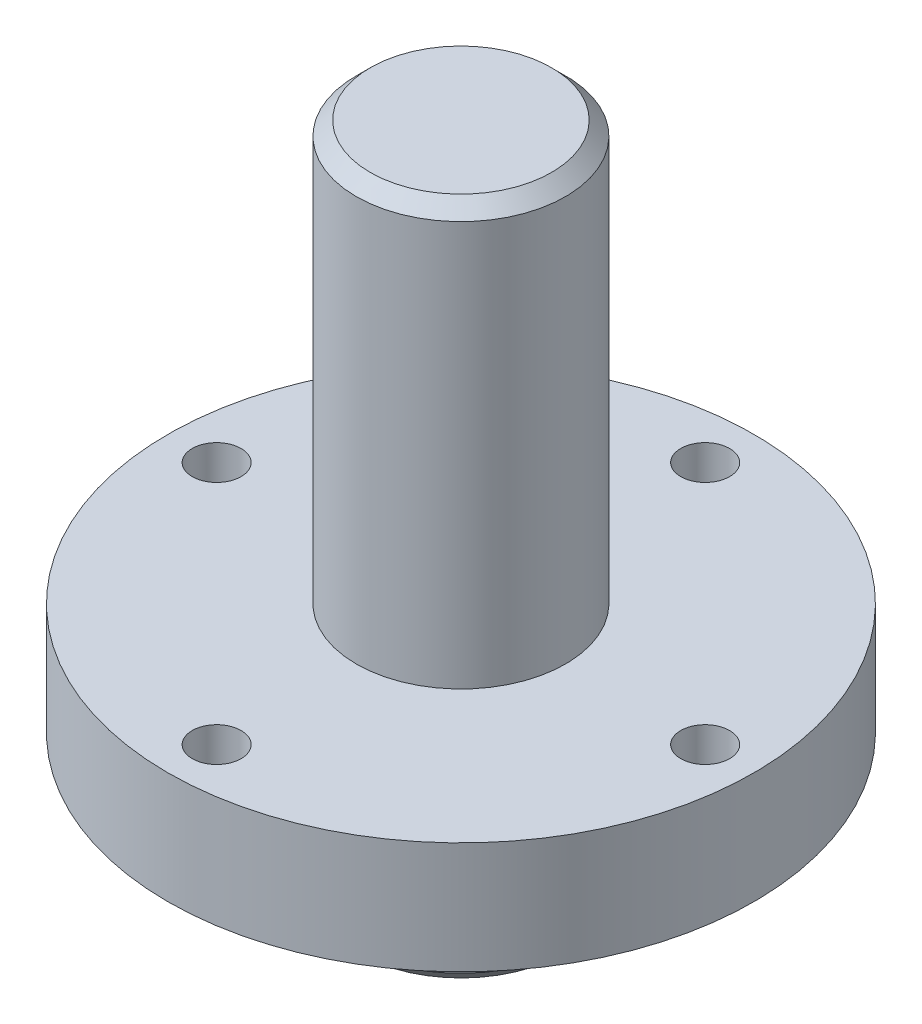
from build123d import *

# Parameters (mm, degrees)
SKETCH1_R           = 15
BOSS_EXTRUDE1_DEPTH = 65
SKETCH2_R           = 14
BOSS_EXTRUDE2_DEPTH = 260
SKETCH3_W           = 22.007775422
SKETCH3_H           = 2
CUT_EXTRUDE1_DEPTH  = 22
CIRPATTERN1_COUNT   = 4
SKETCH4_R           = 10.5
BOSS_EXTRUDE3_DEPTH = 30
SKETCH5_R           = 10.3
BOSS_EXTRUDE4_DEPTH = 10
SKETCH6_R           = 10.5
BOSS_EXTRUDE5_DEPTH = 16
CHAMFER1_SIZE       = 8
CHAMFER1_SIZE2      = 1
SKETCH8_R           = 7.5
BOSS_EXTRUDE6_DEPTH = 30
BOSS_EXTRUDE7_START = -8
SKETCH11_R          = 21
SKETCH11_R_2        = 15
BOSS_EXTRUDE7_DEPTH = 8
SKETCH13_R          = 19
CUT_EXTRUDE4_DEPTH  = 373
SKETCH14_R          = 8.4
BOSS_EXTRUDE8_DEPTH = 10
CHAMFER3_SIZE       = 1
SKETCH16_R          = 1.75
CUT_EXTRUDE5_DEPTH  = 43.213741838
CIRPATTERN3_COUNT   = 4


with BuildPart() as part:
    # Sketch1 → Boss-Extrude1 (new body)
    with BuildSketch(Plane(origin=(0, 0, 0), x_dir=(1, 0, 0), z_dir=(0, 1, 0))):
        with Locations(Location((0, 0, 0), (0, 0, 270))):
            Circle(SKETCH1_R)
    extrude(amount=BOSS_EXTRUDE1_DEPTH)

    # Sketch2 → Boss-Extrude2 (add)
    with BuildSketch(Plane.XZ):
        with Locations(Location((0, 0, 0), (0, 0, 90))):
            Circle(SKETCH2_R)
    extrude(amount=BOSS_EXTRUDE2_DEPTH)

    # Sketch3 → Cut-Extrude1 (cut)
    with BuildSketch(Plane.XZ.offset(260)):
        with Locations((0, -14)):
            Rectangle(SKETCH3_W, SKETCH3_H)
        with Locations((0, 14)):
            Rectangle(SKETCH3_W, SKETCH3_H)
    cut_extrude1 = extrude(amount=-CUT_EXTRUDE1_DEPTH, mode=Mode.SUBTRACT)

    # CirPattern1: Cut-Extrude1 ×4 about axis
    cirpattern1_axis = Axis((0, -260, 0), (0, 1, 0))
    for i in range(1, CIRPATTERN1_COUNT):
        add(cut_extrude1.rotate(cirpattern1_axis, i * 360 / CIRPATTERN1_COUNT), mode=Mode.SUBTRACT)

    # Sketch4 → Boss-Extrude3 (add)
    with BuildSketch(Plane.XZ.offset(260)):
        with Locations(Location((0, 0, 0), (0, 0, 270))):
            Circle(SKETCH4_R)
    extrude(amount=BOSS_EXTRUDE3_DEPTH)

    # Sketch5 → Boss-Extrude4 (add)
    with BuildSketch(Plane.XZ.offset(290)):
        with Locations(Location((0, 0, 0), (0, 0, 270))):
            Circle(SKETCH5_R)
    extrude(amount=BOSS_EXTRUDE4_DEPTH)

    # Sketch6 → Boss-Extrude5 (add)
    with BuildSketch(Plane.XZ.offset(300)):
        with Locations(Location((0, 0, 0), (0, 0, 270))):
            Circle(SKETCH6_R)
    extrude(amount=BOSS_EXTRUDE5_DEPTH)

    # Chamfer1
    chamfer1_edges = [part.edges().sort_by_distance(p)[0] for p in [
        (0, -316, 10.5),
    ]]
    chamfer1_side = [part.faces().sort_by_distance(p)[0] for p in [
        (0, -308, 10.5),
    ]]
    chamfer(chamfer1_edges, length=CHAMFER1_SIZE, length2=CHAMFER1_SIZE2, reference=chamfer1_side[0])

    # Sketch8 → Boss-Extrude6 (add)
    with BuildSketch(Plane(origin=(0, 65, 0), x_dir=(1, 0, 0), z_dir=(0, 1, 0))):
        with Locations(Location((0, 0, 0), (0, 0, 270))):
            Circle(SKETCH8_R)
    extrude(amount=BOSS_EXTRUDE6_DEPTH)

    # Sketch11 → Boss-Extrude7 (add)
    with BuildSketch(Plane(origin=(0, 65, 0), x_dir=(1, 0, 0), z_dir=(0, 1, 0)).offset(BOSS_EXTRUDE7_START)):
        with Locations(Location((0, 0, 0), (0, 0, 270))):
            Circle(SKETCH11_R)
        with Locations(Location((0, 0, 0), (0, 0, 270))):
            Circle(SKETCH11_R_2, mode=Mode.SUBTRACT)
    extrude(amount=BOSS_EXTRUDE7_DEPTH)

    # Sketch13 → Cut-Extrude4 (cut)
    with BuildSketch(Plane.XZ.offset(316)):
        Circle(SKETCH13_R)
    extrude(amount=-CUT_EXTRUDE4_DEPTH, mode=Mode.SUBTRACT)

    # Sketch14 → Boss-Extrude8 (add)
    with BuildSketch(Plane.XZ.offset(-57)):
        with Locations(Location((0, 0, 0), (0, 0, 90))):
            Circle(SKETCH14_R)
    extrude(amount=BOSS_EXTRUDE8_DEPTH)

    # Chamfer3
    chamfer3_edges = [part.edges().sort_by_distance(p)[0] for p in [
        (0, 95, -7.5),
        (0, 47, -8.4),
    ]]
    chamfer(chamfer3_edges, length=CHAMFER3_SIZE)

    # Sketch16 → Cut-Extrude5 (cut, through all)
    with BuildSketch(Plane(origin=(0, 65, 0), x_dir=(1, 0, 0), z_dir=(0, 1, 0))):
        with Locations(Location((17.5, 0, 0), (0, 0, 270))):
            Circle(SKETCH16_R)
    cut_extrude5 = extrude(amount=-CUT_EXTRUDE5_DEPTH, mode=Mode.SUBTRACT)

    # CirPattern3: Cut-Extrude5 ×4 about axis
    cirpattern3_axis = Axis((0, 0, 0), (0, 1, 0))
    for i in range(1, CIRPATTERN3_COUNT):
        add(cut_extrude5.rotate(cirpattern3_axis, i * 360 / CIRPATTERN3_COUNT), mode=Mode.SUBTRACT)


solid = part.part
